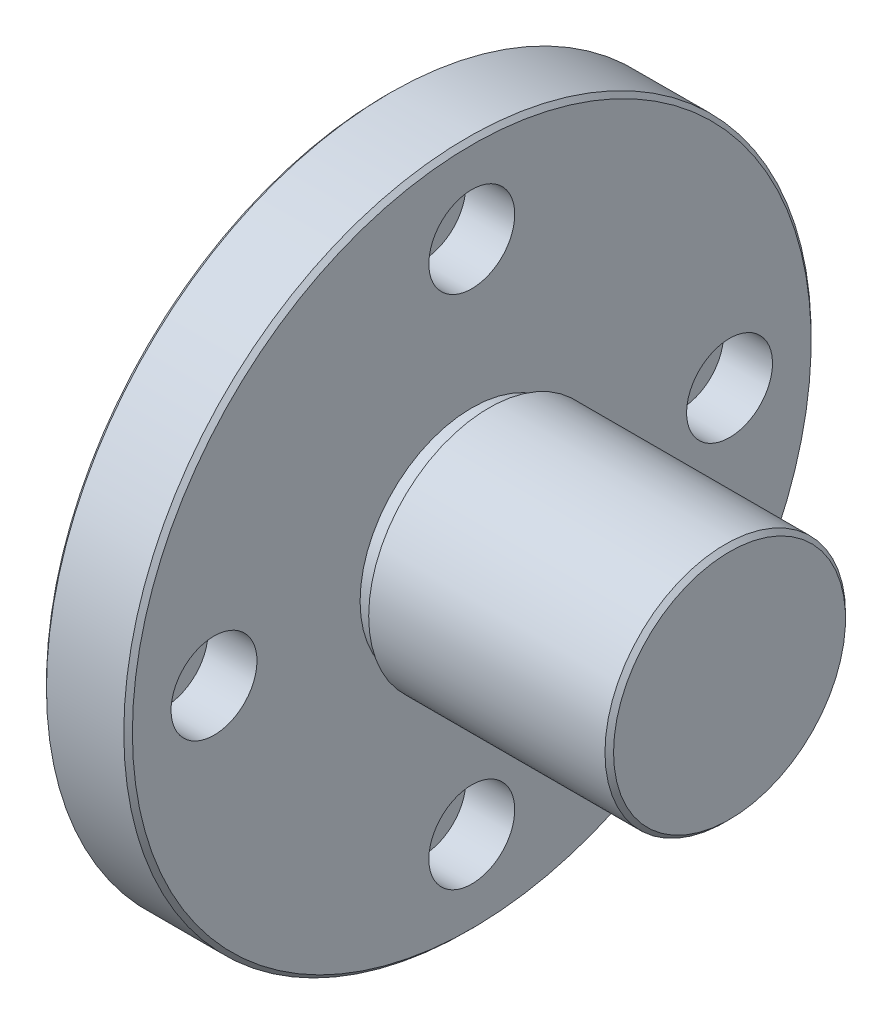
from build123d import *

# Parameters (mm, degrees)
CHAMFER_1_SIZE           = 0.5
PATTERN_CIRCULAR_1_COUNT = 4


with BuildPart() as part:
    # 草图2 → 旋转1 (revolve)
    with BuildSketch(Plane.XY, mode=Mode.PRIVATE) as revolve_1_sk:
        Polygon((0, 0), (0, 40), (10, 40), (10, 13), (12, 13), (12, 14), (40, 14), (40, 0), align=None)
    revolve(revolve_1_sk.sketch.rotate(Axis((0, 0, 0), (1, 0, 0)), 90), axis=Axis((0, 0, 0), (1, 0, 0)))

    # 倒角1
    chamfer_1_edges = [part.edges().sort_by_distance(p)[0] for p in [
        (40, 0, -14),
        (10, 0, -40),
        (0, 0, -40),
    ]]
    chamfer(chamfer_1_edges, length=CHAMFER_1_SIZE)

    # 草图7 → 打孔尺寸(%根据)内六角圆柱头螺钉的类型1 (revolve, cut)
    with BuildSketch(Plane(origin=(10, 30, 0), x_dir=(0, 0, -1), z_dir=(0, 1, 0))):
        Polygon((0, 0), (0, 13.152366702), (2.75, 11.5), (2.75, 5.7), (5, 5.7), (5, 0), align=None)
    hole_wizard_1 = revolve(axis=Axis((16.35, 30, 0), (-1, 0, 0)), mode=Mode.SUBTRACT)

    # 阵列(圆周)1: 打孔尺寸(%根据)内六角圆柱头螺钉的类型1 ×4 about axis
    pattern_circular_1_axis = Axis((0, 0, 0), (1, 0, 0))
    for i in range(1, PATTERN_CIRCULAR_1_COUNT):
        add(hole_wizard_1.rotate(pattern_circular_1_axis, i * 360 / PATTERN_CIRCULAR_1_COUNT), mode=Mode.SUBTRACT)


solid = part.part
